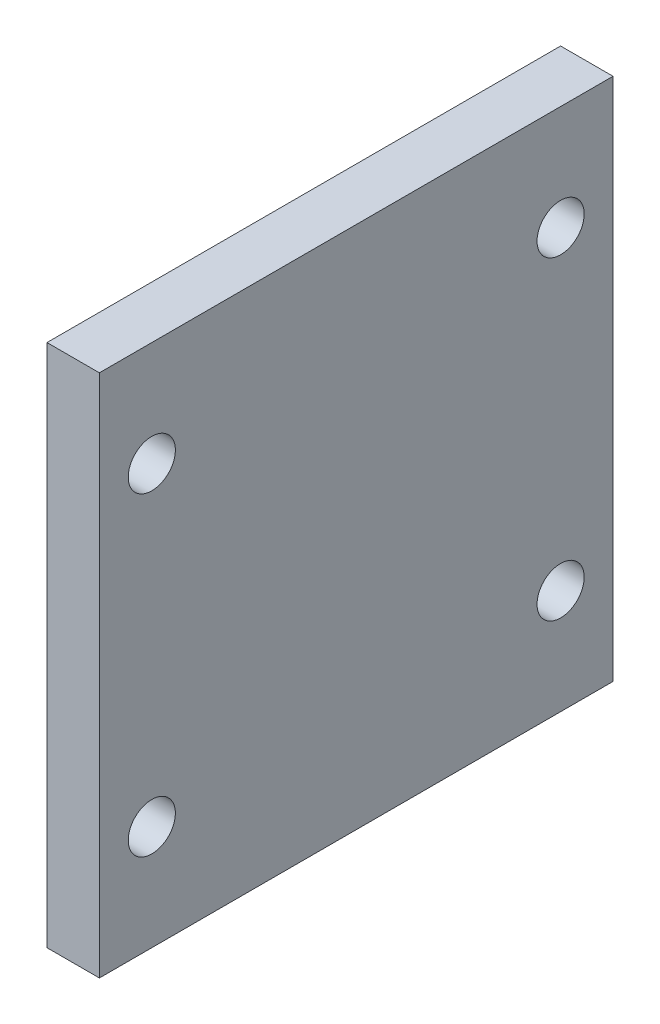
SolidWorks part; units mm, degrees
ref_plane "前视基准面" through (0, 0, 0) normal (0, 0, 1) x (1, 0, 0)
ref_plane "上视基准面" through (0, 0, 0) normal (0, 1, 0) x (1, 0, 0)
ref_plane "右视基准面" through (0, 0, 0) normal (1, 0, 0) x (0, 0, -1)
sketch "草图1" plane through (0, 0, 0) normal (1, 0, 0) x (0, 0, -1)
  line L1 (-49, 50) -> (49, 50)
  line L2 (-49, 50) -> (-49, -50)
  line L3 (-49, -50) -> (49, -50)
  line L4 (49, 50) -> (49, -50)
  line L5 (-49, 50) -> (49, -50) construction
  line L6 (-49, -50) -> (49, 50) construction
  point P0 (0, 0)
  dimension "D1" = 98
  dimension "D2" = 100
extrude "凸台-拉伸1" add sketch "草图1" along normal blind 10
hole_wizard "Ø9.0 (9) 直径孔1" positions "草图2" profile "草图3" hole size "Ø9.0" standard "GB" end condition through all
sketch "草图2" plane through (10, 0, 0) normal (1, 0, 0) x (0, 0, -1)
  line L0 (0, 60.9926) -> (0, 0) construction
  line L1 (0, 0) -> (64.2803, 0) construction
  point P0 (-39, 30)
  point P2 (39, 30)
  point P4 (-39, -30)
  point P6 (39, -30)
  dimension "D1" = 60
  dimension "D2" = 78
sketch "草图3" plane through (10, 30, 39) normal (0, 1, 0) x (0, 0, -1)
  line L0 (0, 0) -> (0, 10)
  line L1 (0, 10) -> (4.5, 10)
  line L2 (4.5, 10) -> (4.5, 0)
  line L5 (4.5, 0) -> (0, 0)
  line L11 (0, -6.35) -> (0, 107.95) construction
  dimension "通孔孔直径" = 9
  dimension "通孔孔深度" = 10
